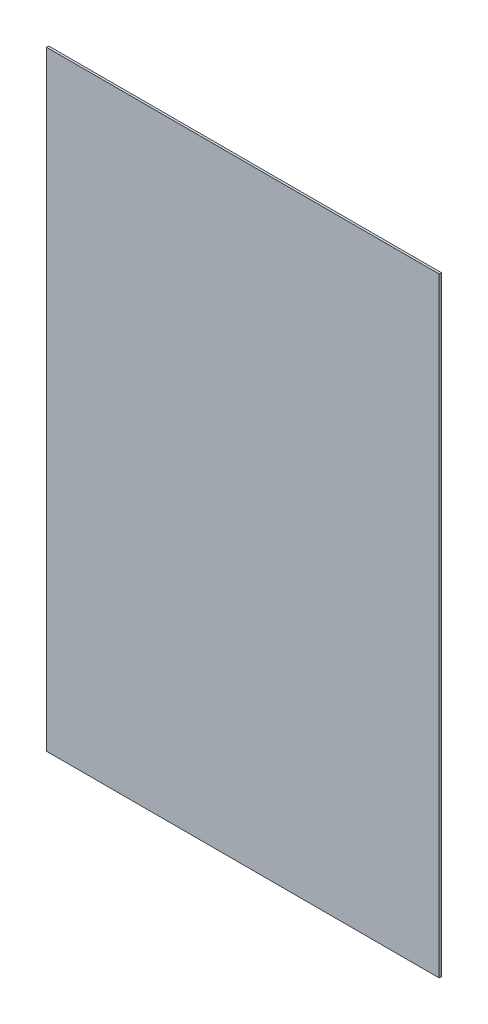
SolidWorks part; units mm, degrees
material "PMMA(有机玻璃)"
ref_plane "前视" through (0, 0, 0) normal (0, 0, 1) x (1, 0, 0)
ref_plane "上视" through (0, 0, 0) normal (0, 1, 0) x (1, 0, 0)
ref_plane "右视" through (0, 0, 0) normal (1, 0, 0) x (0, 0, -1)
sketch "草图1" plane through (0, 0, 0) normal (0, 0, 1) x (1, 0, 0)
  line L1 (-438, 680) -> (438, 680)
  line L2 (-438, 680) -> (-438, -680)
  line L3 (-438, -680) -> (438, -680)
  line L4 (438, 680) -> (438, -680)
  line L5 (-438, 680) -> (438, -680) construction
  line L6 (-438, -680) -> (438, 680) construction
  point P0 (0, 0)
  dimension "D1" = 1360
  dimension "D2" = 876
extrude "凸台-拉伸1" add sketch "草图1" along normal blind 5
hole_wizard "M5 间隙孔1" positions "草图3" profile "草图2" hole size "M5" standard "GB"
sketch "草图3" plane through (0, 0, 5) normal (0, 0, 1) x (1, 0, 0)
  line L0 (-427.5, 273) -> (-427.5, -273) construction
  line L1 (-427.5, -273) -> (427.5, -273) construction
  line L2 (0, 273) -> (0, -273) construction
  line L3 (427.5, 273) -> (-427.5, 273) construction
  line L5 (-427.5, 0) -> (427.5, 0) construction
  line L6 (427.5, -273) -> (427.5, 273) construction
  point P0 (-375, -261)
  point P46 (415.5, 250)
  point P48 (-415.5, 250)
  point P58 (-125, -261)
  point P59 (125, -261)
  point P61 (-125, 261)
  point P62 (125, 261)
  point P64 (-375, 261)
  point P88 (375, -261)
  point P89 (375, 261)
  point P108 (415.5, 0)
  point P109 (-415.5, 0)
  point P110 (415.5, -250)
  point P111 (-415.5, -250)
  dimension "D1" = 12
  dimension "D2" = 12
  dimension "D5" = 3
  dimension "D3" = 12
  dimension "D6" = 4
  dimension "D4" = 2
sketch "草图2" plane through (-375, -261, 5) normal (1, 0, 0) x (0, -1, 0)
  line L0 (0, 0) -> (0, 5)
  line L1 (0, 5) -> (2.75, 5)
  line L2 (2.75, 5) -> (2.75, 0)
  line L5 (2.75, 0) -> (0, 0)
  line L11 (0, -6.35) -> (0, 107.95) construction
  dimension "通孔孔直径" = 5.5
  dimension "通孔孔深度" = 5
